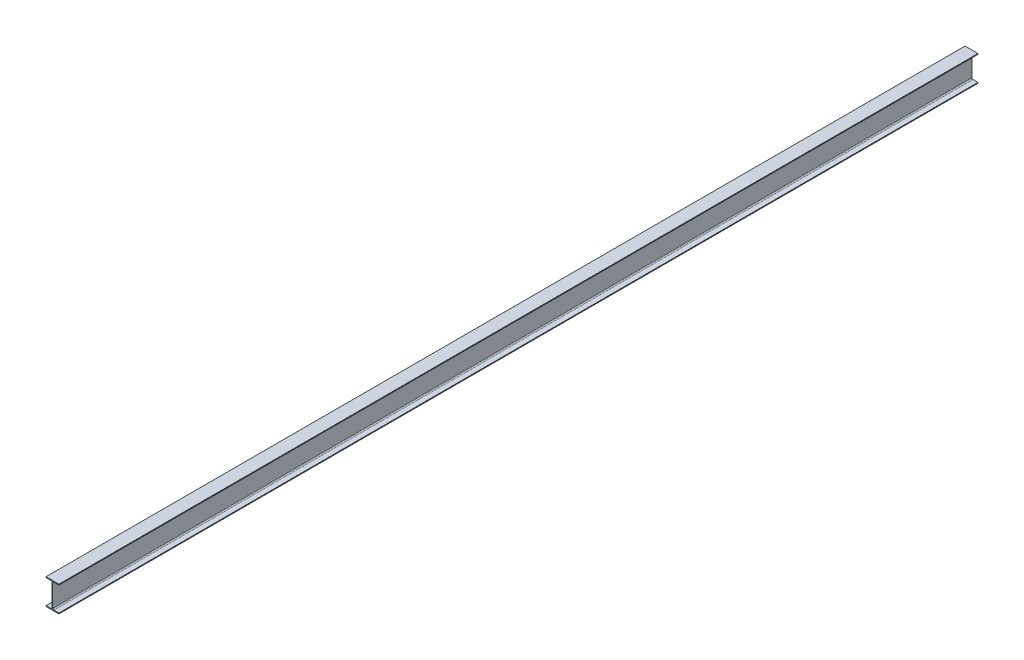
from build123d import *

# Parameters (mm, degrees)
BOSS_EXTRUDE1_DEPTH = 10687


with BuildPart() as part:
    # Sketch1 → Boss-Extrude1 (new body)
    with BuildSketch(Plane.XY):
        with BuildLine():
            Line((75, 0), (-75, 0))
            Line((-75, 0), (-75, 9))
            Line((-75, 9), (-16.25, 9))
            ThreePointArc((-16.25, 9), (-7.057611845, 12.807611845), (-3.25, 22))
            Line((-3.25, 22), (-3.25, 278))
            ThreePointArc((-3.25, 278), (-7.057611845, 287.192388155), (-16.25, 291))
            Line((-16.25, 291), (-75, 291))
            Line((-75, 291), (-75, 300))
            Line((-75, 300), (75, 300))
            Line((75, 300), (75, 291))
            Line((75, 291), (16.25, 291))
            ThreePointArc((16.25, 291), (7.057611845, 287.192388155), (3.25, 278))
            Line((3.25, 278), (3.25, 22))
            ThreePointArc((3.25, 22), (7.057611845, 12.807611845), (16.25, 9))
            Line((16.25, 9), (75, 9))
            Line((75, 9), (75, 0))
        make_face()
    extrude(amount=BOSS_EXTRUDE1_DEPTH)


solid = part.part
